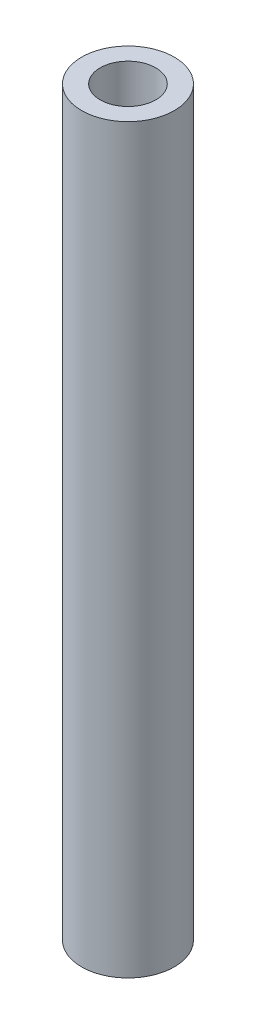
SolidWorks part; units mm, degrees
material "6061 合金"
ref_plane "前视基准面" through (0, 0, 0) normal (0, 0, 1) x (1, 0, 0)
ref_plane "上视基准面" through (0, 0, 0) normal (0, 1, 0) x (1, 0, 0)
ref_plane "右视基准面" through (0, 0, 0) normal (1, 0, 0) x (0, 0, -1)
other "Configuration Table"
sketch "草图1" plane through (0, 0, 0) normal (0, 1, 0) x (1, 0, 0)
  circle A0 centre (0, 0) radius 2.5
  circle A1 centre (0, 0) radius 1.5
  dimension "D1" = 5
  dimension "D2" = 3
extrude "凸台-拉伸1" add sketch "草图1" along normal blind 40
